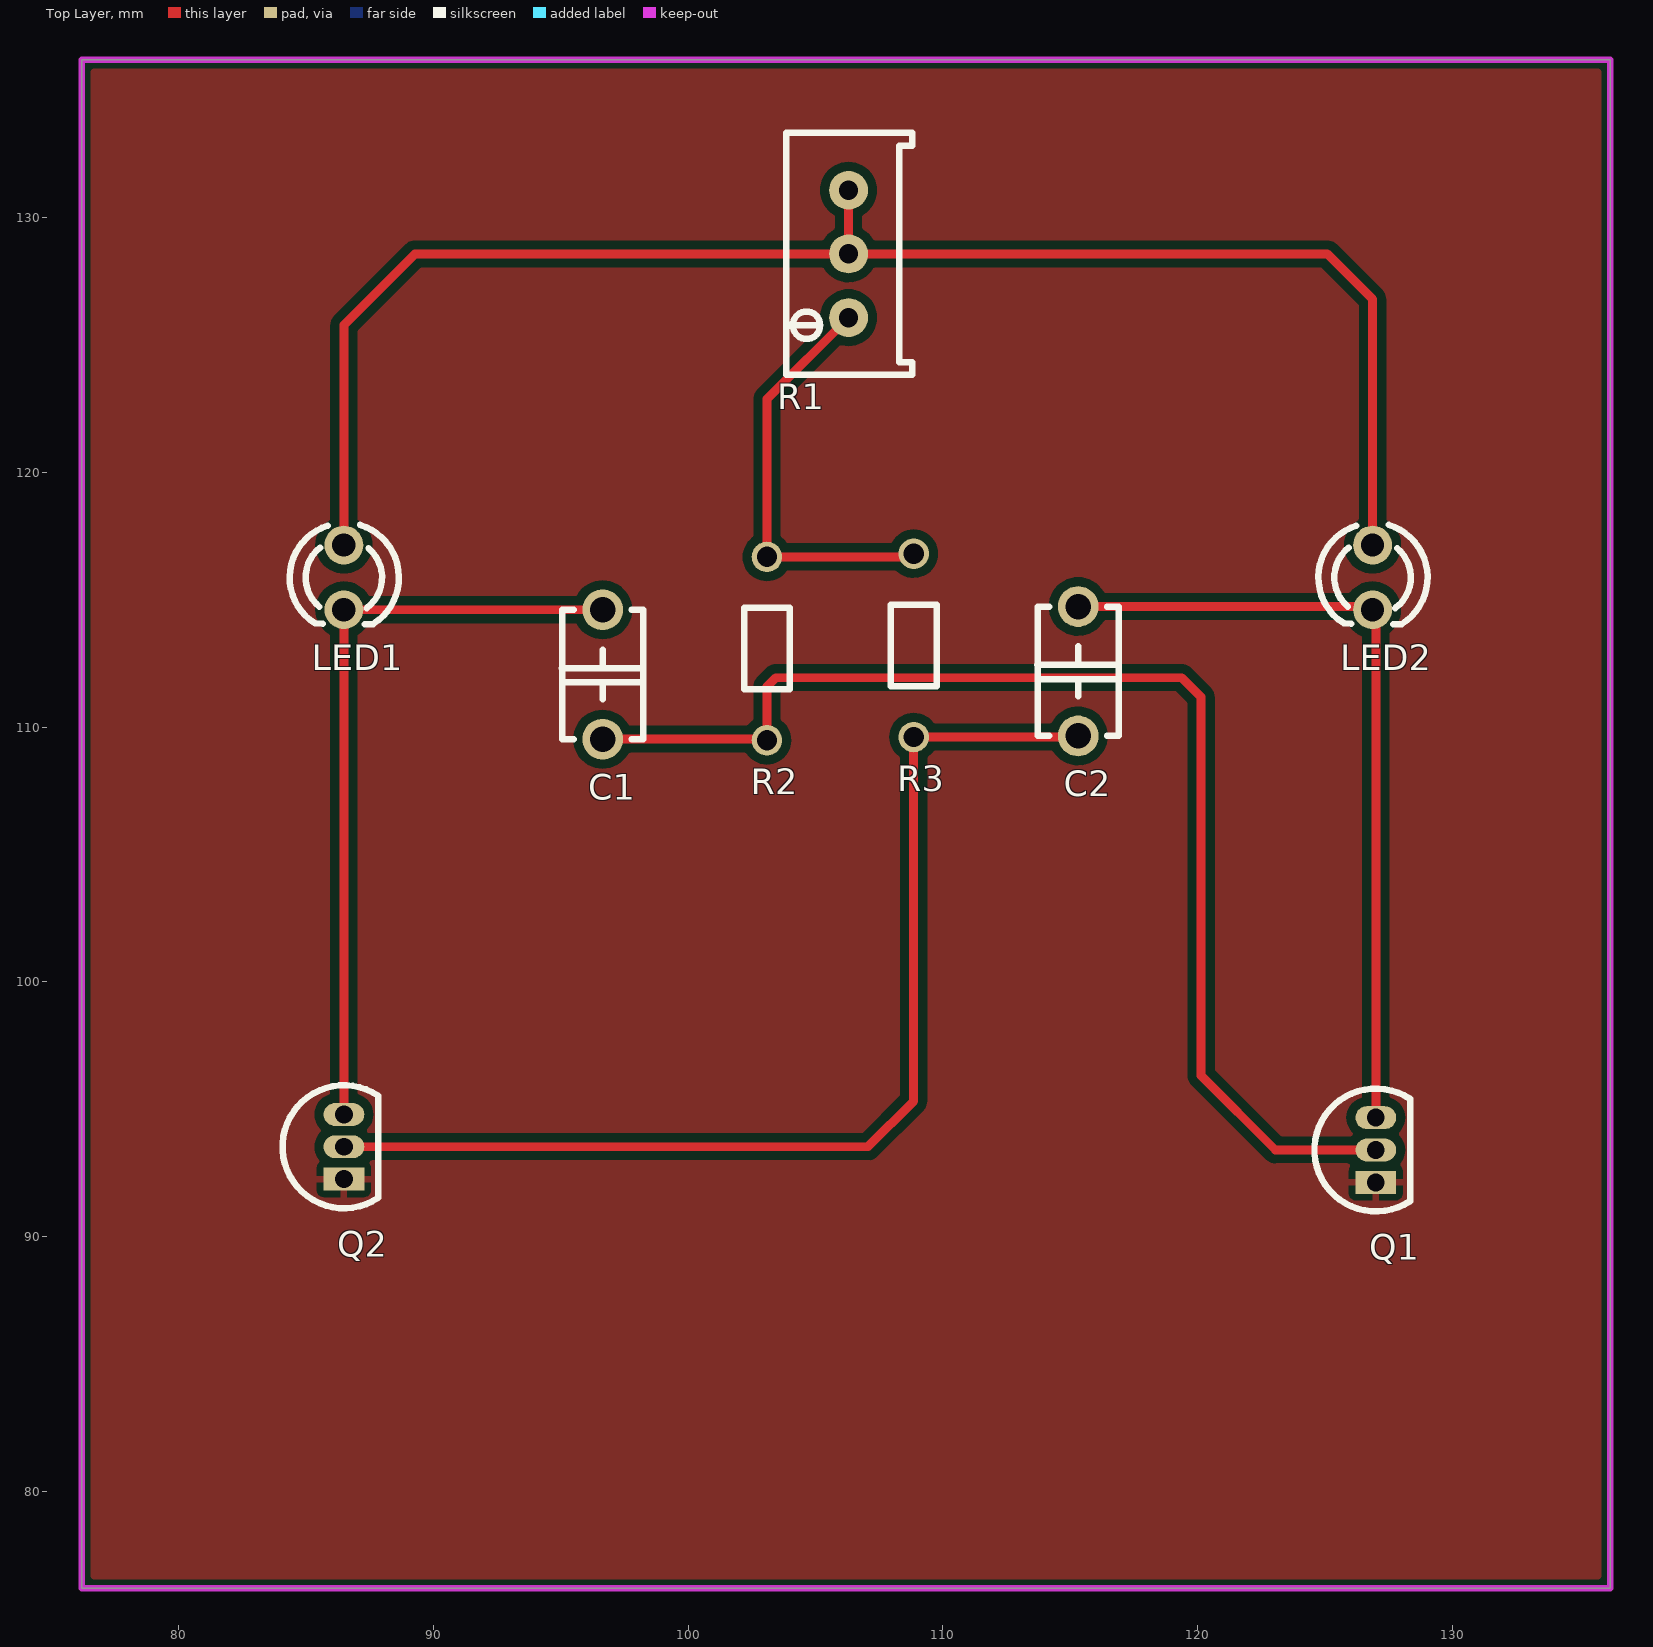
[diagram p0: Top Layer view]
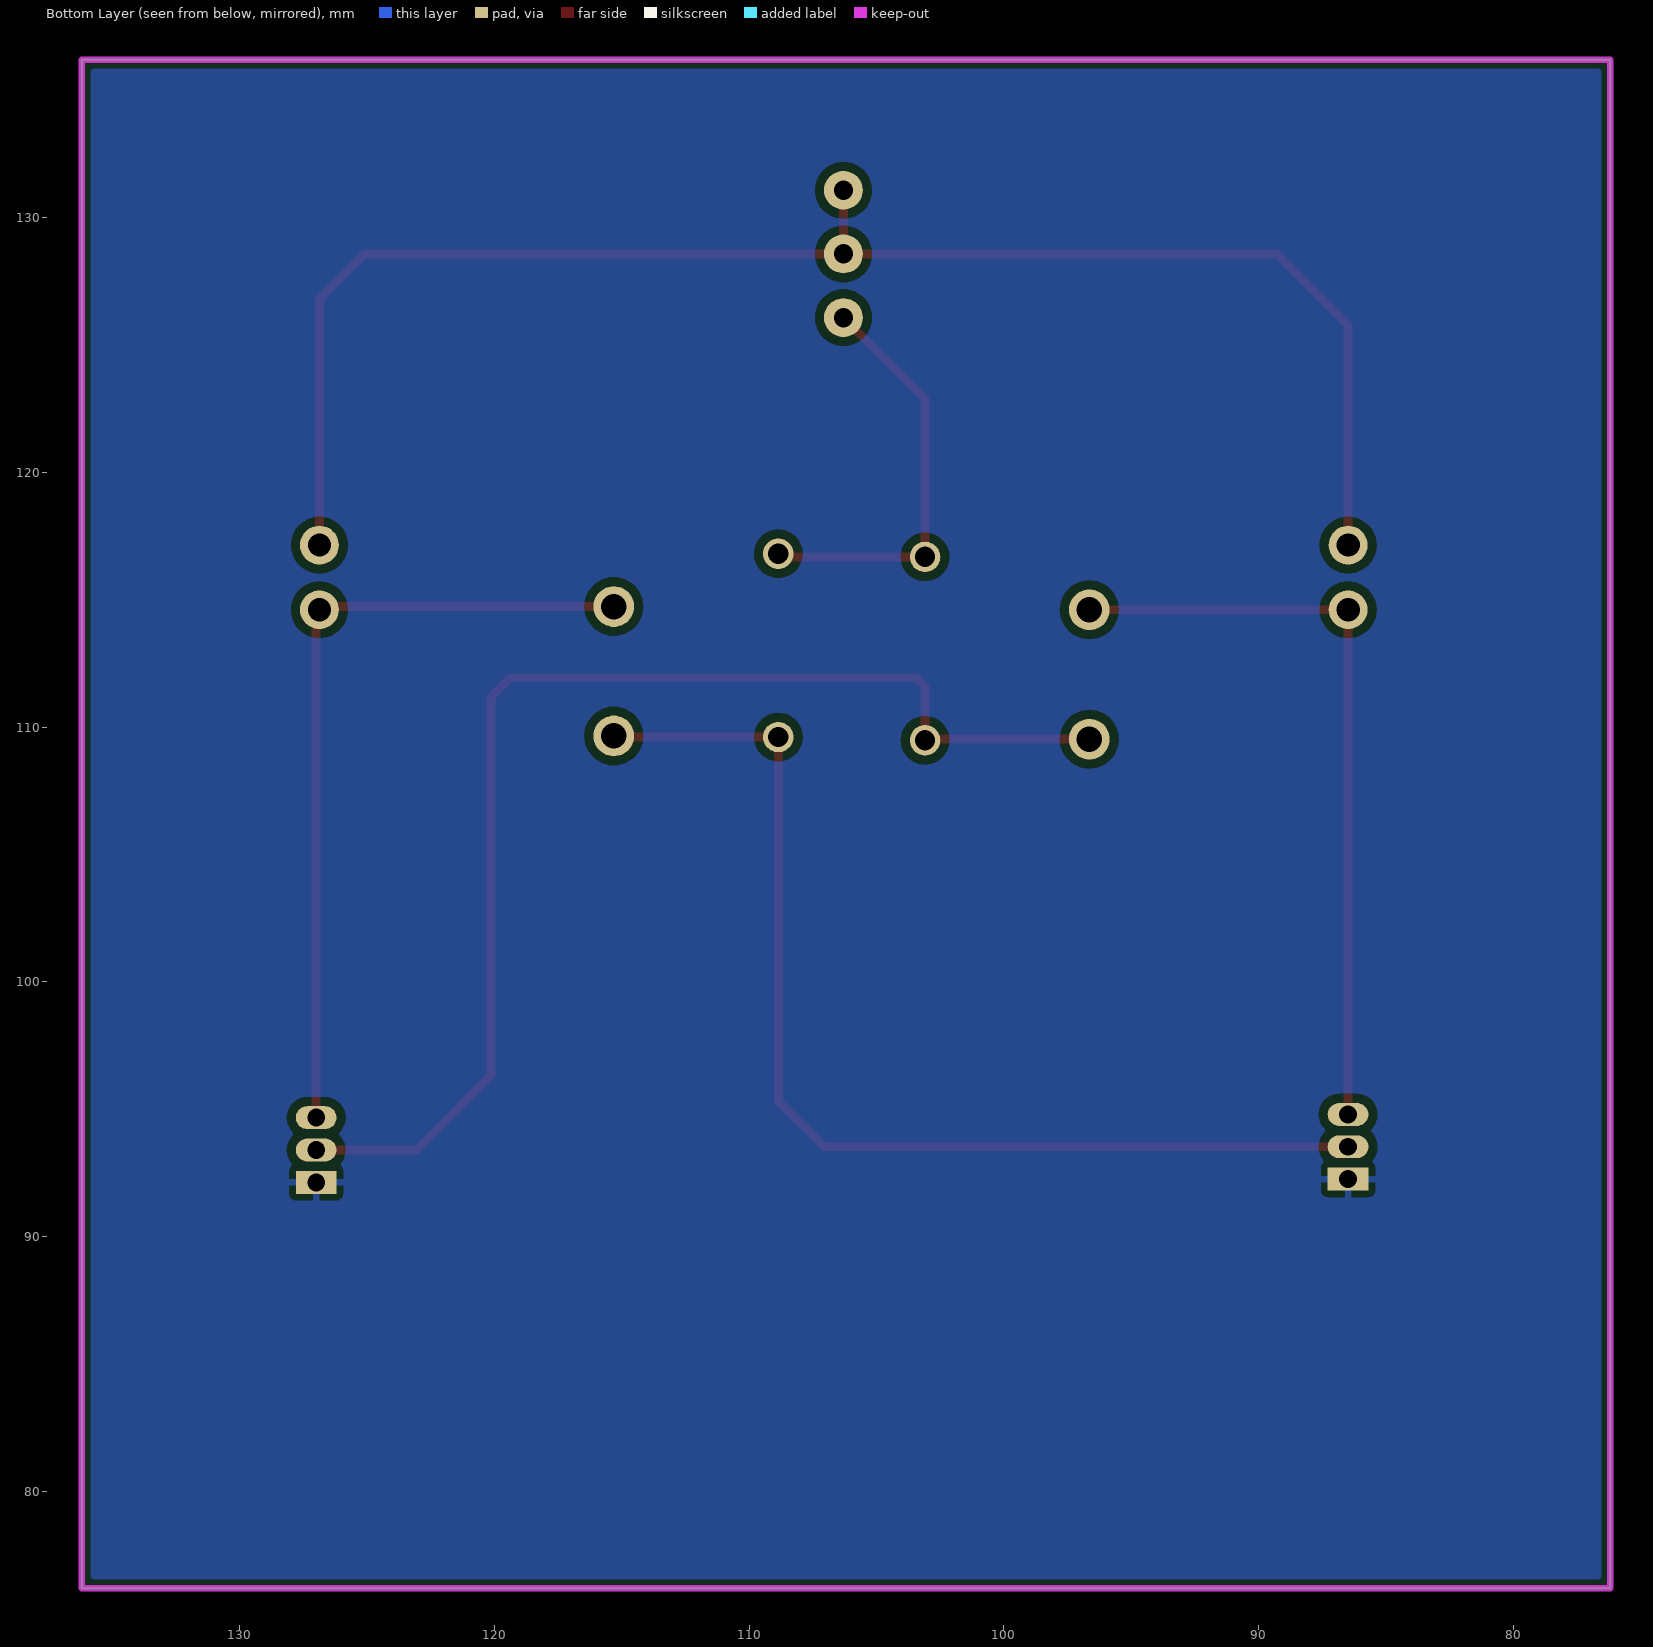
[diagram p1: Bottom Layer view, seen from below]
# Altium PCB MISC52066.pcbdoc
Units mm, origin at the board's own origin, x right, y up, seen from the top; angles counter-clockwise.
Board outline 60 x 60 mm, 2 copper layers (Top Layer, Bottom Layer), stack 1.58 mm thick; 9 components, 7 nets, 21 pads, 0 vias.

## Layer stack, top to bottom
Top Solder Mask Layer: solder mask 0.01, Dk 3.3
Top Layer: signal copper 0.035
Dielectric1: surface 1.51, FR4, Dk 4.5
Bottom Layer: signal copper 0.035
Bottom Solder Mask Layer: solder mask 0.01, Dk 3.3

## Board outline
76.2,136.2 76.2,76.2 136.2,76.2 136.2,136.2

## Design rules (kind name [scope] priority, off if disabled: settings)
BoardOutlineClearance copperThickness2oz_1 [All] p2 off: genericclearance=0.203 ignorepadtopadclearanceinfootprint=FALSE except(0: Arc-SplitContinuation Track-SplitContinuation SMDPad-SplitContinuation THPad-SplitContinuation Via-SplitContinuation Fill-SplitContinuation Region-SplitContinuation Poly-SplitContinuation Text-SplitContinuation Hole-SplitContinuation; 0.152: Arc-CutoutEdge SMDPad-CutoutEdge THPad-CutoutEdge Via-CutoutEdge Fill-CutoutEdge Region-CutoutEdge Text-CutoutEdge; 0.176: Hole-OutlineEdge Hole-CutoutEdge; 0.254: Poly-OutlineEdge Poly-CutoutEdge; 0.3: Arc-OutlineEdge Track-OutlineEdge SMDPad-OutlineEdge THPad-OutlineEdge Via-OutlineEdge Fill-OutlineEdge Region-OutlineEdge Text-OutlineEdge Track-CutoutEdge)
BoardOutlineClearance copperThickness1oz_1 [All] p4: genericclearance=0.25 ignorepadtopadclearanceinfootprint=FALSE except(0: Arc-SplitContinuation Track-SplitContinuation SMDPad-SplitContinuation THPad-SplitContinuation Via-SplitContinuation Fill-SplitContinuation Region-SplitContinuation Poly-SplitContinuation Text-SplitContinuation Hole-SplitContinuation; 0.152: SMDPad-CutoutEdge THPad-CutoutEdge Via-CutoutEdge Fill-CutoutEdge Region-CutoutEdge Text-CutoutEdge; 0.176: Hole-OutlineEdge Hole-CutoutEdge; 0.3: Arc-OutlineEdge Track-OutlineEdge SMDPad-OutlineEdge THPad-OutlineEdge Via-OutlineEdge Fill-OutlineEdge Region-OutlineEdge Text-OutlineEdge Arc-CutoutEdge Track-CutoutEdge; 0.35: Poly-OutlineEdge Poly-CutoutEdge)
Clearance copperThickness2oz [All] p1 off: gap=0.203 ignorepadtopadclearanceinfootprint=FALSE except(0.152: SMDPad-Track SMDPad-SMDPad THPad-Track SMDPad-THPad THPad-THPad Track-Via SMDPad-Via THPad-Via Via-Via Fill-Track Region-Track Fill-SMDPad Region-SMDPad Fill-THPad Region-THPad Fill-Via Region-Via Fill-Fill Fill-Region Region-Region Arc-Track Arc-SMDPad Arc-THPad Arc-Via Fill-Arc Region-Arc Arc-Arc Text-Track SMDPad-Text Text-THPad Text-Via Fill-Text Region-Text Arc-Text Text-Text; 0.176: Hole-Track Hole-SMDPad Hole-THPad Hole-Via Fill-Hole Region-Hole Hole-Arc Hole-Text; 0.254: Poly-Track Poly-SMDPad Poly-THPad Poly-Via Poly-Fill Poly-Region Poly-Poly Poly-Arc Poly-Text Poly-Hole)
Clearance copperThickness1oz [All] p3: gap=0.25 ignorepadtopadclearanceinfootprint=FALSE except(0.152: SMDPad-Track SMDPad-SMDPad THPad-Track SMDPad-THPad THPad-THPad Track-Via SMDPad-Via THPad-Via Via-Via Fill-Track Region-Track Fill-SMDPad Region-SMDPad Fill-THPad Region-THPad Fill-Via Region-Via Fill-Fill Fill-Region Region-Region Arc-Track Arc-SMDPad Arc-THPad Arc-Via Fill-Arc Region-Arc Arc-Arc Text-Track SMDPad-Text Text-THPad Text-Via Fill-Text Region-Text Arc-Text Text-Text; 0.176: Hole-Track Hole-SMDPad Hole-THPad Hole-Via Fill-Hole Region-Hole Hole-Arc Hole-Text; 0.35: Poly-Track Poly-SMDPad Poly-THPad Poly-Via Poly-Fill Poly-Region Poly-Poly Poly-Arc Poly-Text Poly-Hole)
Creepage creepage [All] p1: checkdistance=0 ignoreinternallayers=TRUE applytopolygonpour=TRUE
DiffPairsRouting differentialPair [All] p1: maxlimit=0.152 minlimit=0.152 mostfreqgap=0.152 toplayer_minwidth=0.127 toplayer_prefwidth=0.254 toplayer_maxwidth=2.54 toplayer_mingap=0.152 toplayer_prefgap=0.152 toplayer_maxgap=0.152 bottomlayer_minwidth=0.127 bottomlayer_prefwidth=0.254 bottomlayer_maxwidth=2.54 bottomlayer_mingap=0.152 bottomlayer_prefgap=0.152 bottomlayer_maxgap=0.152 maxuncoupledlength=0.254
HoleToHoleClearance otherClearance [All] p1: gap=0.3 allowstackedmicrovias=TRUE
Length netLength [All] p1: minlimit=0 maxlimit=0
MatchedLengths netLengthTolerance [All] p1: tolerance=25.4
PasteMaskExpansion pasteMaskExpansion [All] p1: expansion=0
PlaneConnect innerPlane [All] p1: planeconnectstyle=Relief reliefexpansion=0.508 reliefentries=4 reliefconductorwidth=0.254 reliefairgap=0.254
PolygonConnect copperRegion [(InNet('GND'))] p1: connectstyle=Relief reliefconductorwidth=0.254 reliefentries=4 polygonreliefangle="90 Angle" airgapwidth=0.254 via.connectstyle=Relief via.reliefconductorwidth=0.254 via.reliefentries=4 via.polygonreliefangle="90 Angle" via.airgapwidth=0.254
RoutingVias viaSize [All] p1: holewidth=0.3 width=0.5 viastyle="Through Hole" minholewidth=0.3 minwidth=0.5 maxholewidth=6.3 maxwidth=10
SolderMaskExpansion solderMaskExpansion [IsVia] p1: expansion=-25.4 istentingtop=TRUE
SolderMaskExpansion solderMaskExpansion [All] p2: expansion=0.051 istentingtop=FALSE
Width copperThickness2oz_2 [All] p1 off: maxlimit=2.54 minlimit=0.203 preferedwidth=0.254
Width copperThickness1oz_2 [All] p2: maxlimit=0.254 minlimit=0.254 preferedwidth=0.254 toplayer_minwidth=0.351 toplayer_maxwidth=2.54 toplayer_prefwidth=0.351 bottomlayer_minwidth=0.351 bottomlayer_maxwidth=2.54 bottomlayer_prefwidth=0.351

## Components (designator, comment, footprint, x,y, rotation, side; value= is the part's Value field where it differs from the comment)
C1 "100uF" CAP-TH_L5.1-W3.2-P5.08-D0.50 96.647,112.07 r270 top
C2 "100uF" CAP-TH_L5.1-W3.2-P5.08-D0.50 115.316,112.197 r270 top
LED1 "" LED_TH-3mm 86.487,115.88 r270 top
LED2 "" LED_TH-3mm 126.873,115.88 r270 top
Q1 "" S8050_TO_92 127,93.401 r90 top
Q2 "" S8050_TO_92 86.487,93.528 r90 top
R1 "10k" R_3296 106.172,128.58 r90 top
R2 "10k" Res_1/8W 103.16,113.086 r90 top
R3 "10k" Res_1/8W 108.919,113.213 r90 top

## Footprints (in the part's own frame and the unit in brackets; to place one, negate y for a bottom-side part, rotate by r counter-clockwise, add the part's x,y. Pads: shape width x height; smd on the part's side, far side on the other; paste and mask are expansions set on the pad)
CAP-TH_L5.1-W3.2-P5.08-D0.50 [mm]
  round 1.6 hole 1 paste+0 mask+0.05: 1(-2.54,0) 2(2.54,0)
  silkscreen extent -2.54,-1.6 2.54,1.59
LED_TH-3mm [mil]
  round 60 hole 36 paste+0 mask+2: 1(-50,0) 2(50,0)
  silkscreen extent -81,-84 72,85
R_3296 [mil]
  round 60 hole 30 paste+0 mask+2: 1(-98.4,-5) 2(0,-5) 3(98.4,-5)
  silkscreen extent -187,-103 187,92
Res_1/8W [mil]
  round 47.2 hole 31.5 paste+0 mask+2: 1(-141.7,2.48) 2(141.7,2.48)
  silkscreen extent -63,-33 63,38
S8050_TO_92 [mil]
  rect 35.4x63 hole 27.6 paste+0 mask+2: 1(-50,0)
  oval 35.4x63 hole 27.6 paste+0 mask+2: 2(0,0) 3(50,0)
  silkscreen extent -95,-53 95,95

## Nets (pads, with @x,y where several pads share a name; then routed paths per layer and width w, separated by ;. In a path a pad name is that pad's centre, name@x,y a point inside that pad or via, vN(x,y) a via of type N, cw(c..) or ccw(c..) an arc to the next point about the centre after c; other vN are vias at no path point)
$1N1: R1.1 R2.2 R3.2 | length 16.5
  Top Layer w0.35: R1.1 103.097,122.879 R2.2 108.729,116.685 R3.2
$1N4: C1.2 Q1.2 R2.1 | length 49
  Top Layer w0.35: C1.2 103.054,109.53 R2.1 103.097,111.593 103.447,111.943 119.38,111.943 120.142,111.181 120.142,96.322 123.063,93.401 Q1.2
$1N5: C2.2 Q2.2 R3.1 | length 43.9
  Top Layer w0.35: Q2.2 107.061,93.528 108.856,95.323 R3.1 115.273,109.614 C2.2
$1N7: C1.1 LED1.2 Q2.3 | length 30
  Top Layer w0.35: Q2.3 LED1.2 C1.1
$1N8: C2.1 LED2.2 Q1.3 | length 31.6
  Top Layer w0.35: C2.1 126.746,114.737 LED2.2 127,114.483 Q1.3
+12V: LED1.1 LED2.1 R1.2 R1.3 | length 63.1
  Top Layer w0.35: LED1.1 86.487,125.786 89.281,128.58 R1.2 ; R1.3 R1.2 ; LED2.1 126.873,126.802 125.095,128.58 R1.2
GND: Q1.1 Q2.1

## Polygon pours and split planes (outlines as drawn)
GND on Top Layer (solid, remove dead copper, pour order 0): 76.2,136.2 76.2,76.2 136.2,76.2 136.2,136.2
GND on Bottom Layer (solid, remove dead copper, pour order 2): 76.2,136.2 76.2,76.2 136.2,76.2 136.2,136.2

## Keep-outs
Board Outline Layer:
  the board outline again, w0.254